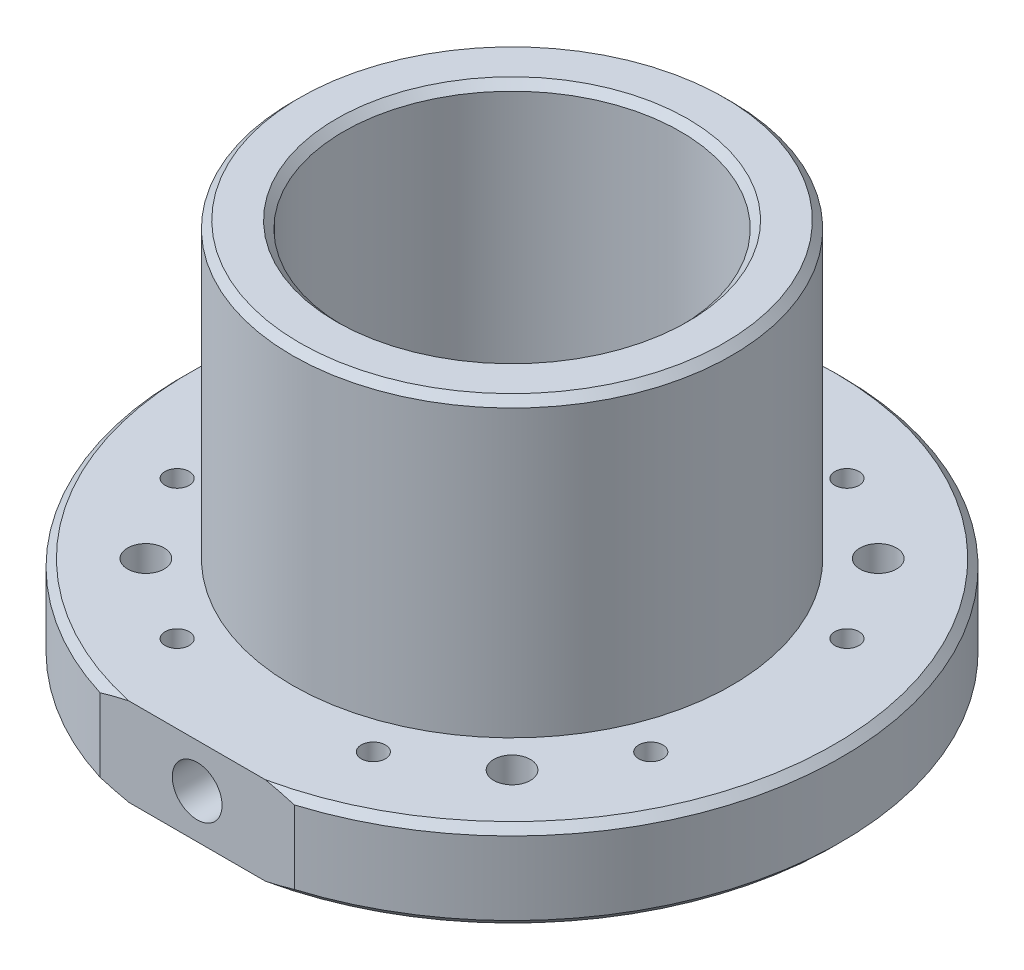
SolidWorks part; units mm, degrees
ref_plane "Front Plane" through (0, 0, 0) normal (0, 0, 1) x (1, 0, 0)
ref_plane "Top Plane" through (0, 0, 0) normal (0, 1, 0) x (1, 0, 0)
ref_plane "Right Plane" through (0, 0, 0) normal (1, 0, 0) x (0, 0, -1)
sketch "Sketch1" plane through (0, 0, 0) normal (0, 1, 0) x (1, 0, 0)
  circle A0 centre (0, 0) radius 45
  dimension "D1" = 90
extrude "Boss-Extrude1" add sketch "Sketch1" along normal blind 12
sketch "Sketch2" plane through (0, 12, 0) normal (0, 1, 0) x (1, 0, 0)
  circle A0 centre (0, 0) radius 30
  dimension "D1" = 60
extrude "Boss-Extrude2" add sketch "Sketch2" along normal blind 40
cosmetic thread "Cosmetic Thread1" parameters "D1"=15, "D2"=58.5
sketch "Sketch3" plane through (0, 0, 0) normal (0, -1, 0) x (1, 0, 0)
  circle A0 centre (0, 0) radius 23
  dimension "D1" = 46
extrude "Cut-Extrude1" cut sketch "Sketch3" against normal through all
chamfer "Chamfer1" distance 1 angle 45 5 edges at (0, 0, 45) (0, 12, 45) (0, 52, 30) (0, 52, -23) (0, 0, -23)
hole_wizard "M6 Tapped Hole1" positions "Sketch5" profile "Sketch4" tap size "M6" standard "Gb" end condition through all
sketch "Sketch5" plane through (0, 0, 0) normal (0, -1, 0) x (-1, 0, 0)
  line L0 (0, 0) -> (0, -37.1797) construction
  line L2 (0, 0) -> (-51.8806, 0) construction
  point P0 (25, -25)
  point P2 (-25, -25)
  point P4 (-25, 25)
  point P6 (25, 25)
  dimension "D1" = 50
  dimension "D2" = 50
sketch "Sketch4" plane through (-25, 0, 25) normal (1, 0, 0) x (0, 0, -1)
  line L0 (0, 0) -> (0, 52)
  line L1 (0, 52) -> (2.5, 52)
  line L2 (2.5, 52) -> (2.5, 0)
  line L5 (2.5, 0) -> (0, 0)
  line L11 (0, -6.35) -> (0, 107.95) construction
  dimension "通孔螺纹孔钻头直径" = 5
  dimension "通孔螺纹孔钻头深度" = 52
cosmetic thread "Hole Cosmetic Thread1" parameters "D2"=6
cosmetic thread "Hole Cosmetic Thread2" parameters "D2"=6
cosmetic thread "Hole Cosmetic Thread3" parameters "D2"=6
cosmetic thread "Hole Cosmetic Thread4" parameters "D2"=6
hole_wizard "M4 Tapped Hole1" positions "Sketch7" profile "Sketch6" tap size "M4" standard "Gb" end condition through all
sketch "Sketch7" plane through (0, 0, 0) normal (0, -1, 0) x (-1, 0, 0)
  line L4 (0, 0) -> (0, -45) construction
  line L6 (0, 0) -> (17.2208, -41.5746) construction
  circle A0 centre (0, 0) radius 45 construction
  circle A1 centre (0, 0) radius 35 construction
  point P4 (13.3939, -32.3358)
  dimension "D2" = 70
  dimension "D1" = 22.5
sketch "Sketch6" plane through (-13.3939, 0, 32.3358) normal (1, 0, 0) x (0, 0, -1)
  line L0 (0, 0) -> (0, 52)
  line L1 (0, 52) -> (1.65, 52)
  line L2 (1.65, 52) -> (1.65, 0)
  line L5 (1.65, 0) -> (0, 0)
  line L11 (0, -6.35) -> (0, 107.95) construction
  dimension "通孔螺纹孔钻头直径" = 3.3
  dimension "通孔螺纹孔钻头深度" = 52
cosmetic thread "Hole Cosmetic Thread6" parameters "D2"=4
sketch "Sketch8" plane through (0, 0, 0) normal (0, -1, 0) x (1, 0, 0)
  line L0 (-13.2665, 43) -> (13.2665, 43)
  circle A1 centre (0, 0) radius 45 construction
  arc A2 (13.2665, 43) -> (-13.2665, 43) centre (0, 0) ccw
  dimension "D1" = 43
extrude "Cut-Extrude2" cut sketch "Sketch8" against normal through all
pattern_circular "CirPattern1" count 8 over 360 about axis through (0, 0, 0) along (0, 1, 0) of "M4 Tapped Hole1"
hole_wizard "M8 Tapped Hole1" positions "Sketch10" profile "Sketch9" tap size "M8" standard "Gb"
sketch "Sketch10" plane through (0, 0, 43) normal (0, 0, 1) x (1, 0, 0)
  line L0 (-44, 0) -> (44, 0) construction
  point P0 (0, 6)
  dimension "D1" = 6
sketch "Sketch9" plane through (0, 6, 43) normal (1, 0, 0) x (0, -1, 0)
  line L0 (0, 0) -> (0, 20)
  line L1 (0, 20) -> (3.4, 20)
  line L2 (3.4, 20) -> (3.4, 0)
  line L5 (3.4, 0) -> (0, 0)
  line L11 (0, -6.35) -> (0, 107.95) construction
  dimension "通孔螺纹孔钻头直径" = 6.8
  dimension "通孔螺纹孔钻头深度" = 20
cosmetic thread "Hole Cosmetic Thread9" parameters "D2"=8
